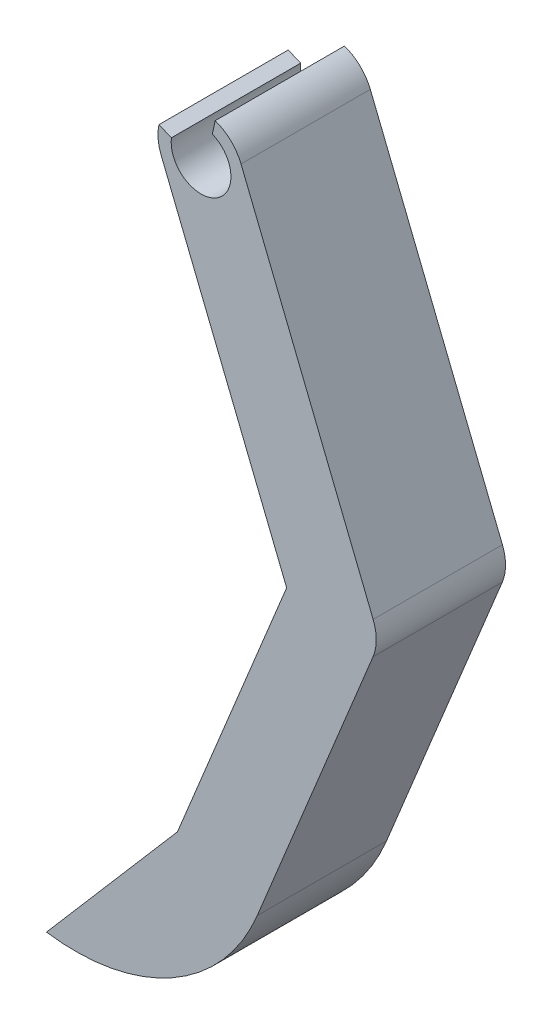
from build123d import *

# Parameters (mm, degrees)
BOSS_EXTRUDE1_DEPTH = 6


with BuildPart() as part:
    # Sketch1 → Boss-Extrude1 (new body)
    with BuildSketch(Plane.XY):
        with BuildLine():
            Line((23.424737155, -30.334071959), (17.293543757, -15.098809177))
            ThreePointArc((17.293543757, -15.098809177), (16.817822135, -14.397549548), (16.094423456, -13.956221462))
            Line((16.094423456, -13.956221462), (15.963008089, -14.561962892))
            ThreePointArc((15.963008089, -14.561962892), (16.131735441, -17.04624853), (14.064088238, -15.658812373))
            Line((14.064088238, -15.658812373), (13.483620184, -15.421447711))
            ThreePointArc((13.483620184, -15.421447711), (13.445284936, -16.014246024), (13.582760132, -16.592156052))
            Line((13.582760132, -16.592156052), (19.41043004, -31.073200227))
            Line((19.41043004, -31.073200227), (19.719217872, -30.321121581))
            ThreePointArc((19.719217872, -30.321121581), (21.576335078, -29.08075761), (23.424737155, -30.334071959))
        make_face()
        with BuildLine():
            ThreePointArc((23.419472814, -31.840369211), (23.569333129, -31.087735131), (23.424737155, -30.334071959))
            ThreePointArc((23.424737155, -30.334071959), (21.576335078, -29.08075761), (19.719217872, -30.321121581))
            Line((19.719217872, -30.321121581), (19.41043004, -31.073200227))
            Line((19.41043004, -31.073200227), (19.71395353, -31.827418834))
            ThreePointArc((19.71395353, -31.827418834), (21.562355608, -33.080733182), (23.419472814, -31.840369211))
        make_face()
        with BuildLine():
            Line((18.045273154, -44.929682928), (23.419472814, -31.840369211))
            ThreePointArc((23.419472814, -31.840369211), (21.562355608, -33.080733182), (19.71395353, -31.827418834))
            Line((19.71395353, -31.827418834), (19.41043004, -31.073200227))
            Line((19.41043004, -31.073200227), (14.345018212, -43.410435298))
            Line((14.345018212, -43.410435298), (8.266248414, -50.481735298))
            ThreePointArc((8.266248414, -50.481735298), (14.114121661, -49.393703769), (18.045273154, -44.929682928))
        make_face()
    extrude(amount=BOSS_EXTRUDE1_DEPTH)


solid = part.part
